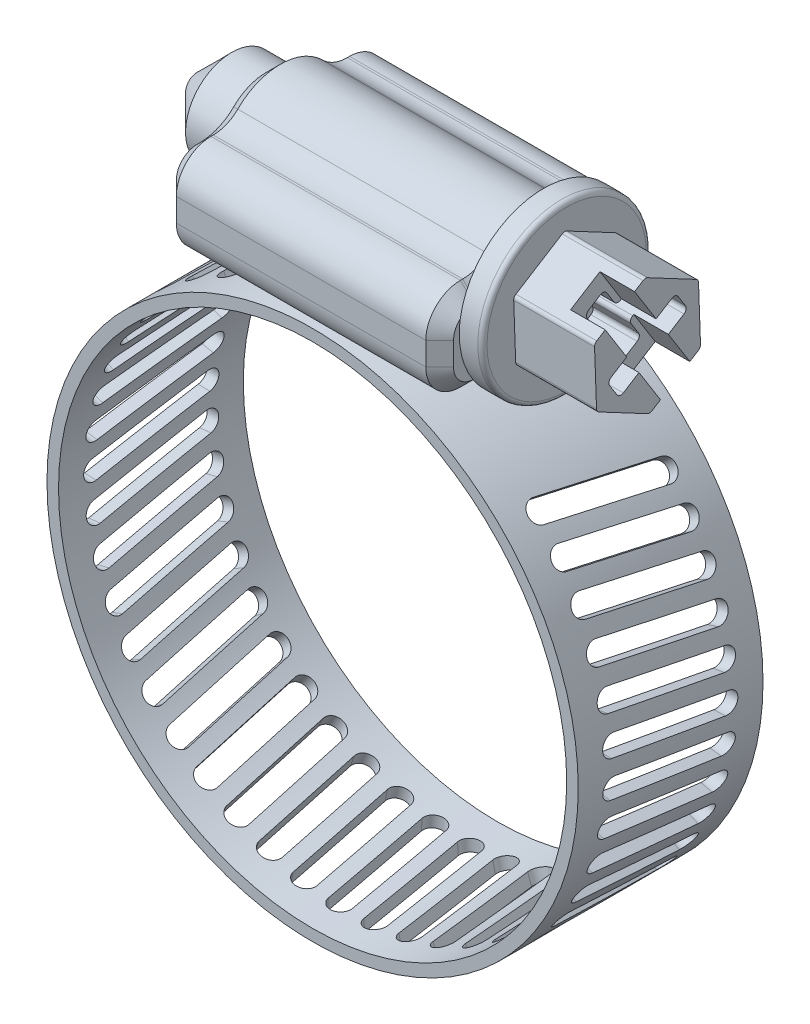
SolidWorks part; units mm, degrees
material "AISI 304"
ref_plane "Front Plane" through (0, 0, 0) normal (0, 0, 1) x (1, 0, 0)
ref_plane "Top Plane" through (0, 0, 0) normal (0, 1, 0) x (1, 0, 0)
ref_plane "Right Plane" through (0, 0, 0) normal (1, 0, 0) x (0, 0, -1)
sketch "Sketch1" plane through (0, 0, 0) normal (0, 0, 1) x (1, 0, 0)
  circle A0 centre (0, 0) radius 11
  dimension "D1" = 22
extrude "Extrude-Thin1" add sketch "Sketch1" along normal blind 8 thin
ref_plane "Plane1" through (0, 11.5, 0) normal (0, 1, 0) x (1, 0, 0)
ref_plane "Plane2" through (0, 0, 0) normal (1, 0, 0) x (0, 0, -1)
ref_plane "Plane3" through (6, 0, 0) normal (1, 0, 0) x (0, 0, -1)
sketch "Sketch2" plane through (6, 0, 0) normal (1, 0, 0) x (0, 0, -1)
  line L0 (-7, 11.5) -> (-1, 11.5)
  line L1 (6.765, 11.5) -> (-6.765, 11.5) construction
  line L2 (0.5, 13) -> (0.5, 14)
  line L3 (-1, 15.5) -> (-1.1, 15.5)
  line L4 (-8.5, 13) -> (-8.5, 14)
  line L5 (-7, 15.5) -> (-6.9, 15.5)
  line L6 (-8, 11.5) -> (-8, -11.5) construction
  line L7 (0, -11.5) -> (0, 11.5) construction
  arc A0 (-2.1608, 15.9395) -> (-5.8392, 15.9395) centre (-4, 14.1007) ccw
  arc A1 (0.5, 13) -> (-1, 11.5) centre (-1, 13) cw
  arc A2 (-8.5, 13) -> (-7, 11.5) centre (-7, 13) ccw
  arc A3 (-7, 15.5) -> (-8.5, 14) centre (-7, 14) ccw
  arc A4 (-1, 15.5) -> (0.5, 14) centre (-1, 14) cw
  arc A5 (-2.1608, 15.9395) -> (-1.1, 15.5) centre (-1.1, 17) ccw
  arc A6 (-5.8392, 15.9395) -> (-6.9, 15.5) centre (-6.9, 17) cw
  point P19 (0.5, 11.5)
  point P22 (-8.5, 11.5)
  dimension "D4" = 1.5
  dimension "D1" = 0.5
  dimension "D2" = 0.5
  dimension "D3" = 4
  dimension "D5" = 0.1
  dimension "D6" = 0.1
extrude "Boss-Extrude1" add sketch "Sketch2" against normal blind 12 separate body
sketch "Sketch3" plane through (6, 0, 0) normal (1, 0, 0) x (0, 0, -1)
  line L1 (-4.0935, 16.6997) -> (-6.2976, 15.3193)
  line L2 (-6.2976, 15.3193) -> (-6.2041, 12.7203)
  line L3 (-6.2041, 12.7203) -> (-3.9065, 11.5017)
  line L4 (-3.9065, 11.5017) -> (-1.7024, 12.8821)
  line L5 (-1.7024, 12.8821) -> (-1.7959, 15.4812)
  line L6 (-1.7959, 15.4812) -> (-4.0935, 16.6997)
  circle A1 centre (-4, 14.1007) radius 2.2523 construction
  arc A2 (-2.1608, 15.9395) -> (-5.8392, 15.9395) centre (-4, 14.1007) ccw construction
extrude "Boss-Extrude2" add sketch "Sketch3" along normal blind 4.5 separate body
chamfer "Chamfer1" distance 0.6 angle 45 24 edges at (6, 11.5, 4) (6, 11.9393, 8.0607) (6, 13.5, 8.5) (6, 15.0607, 8.0607) (6, 15.5, 6.95) (6, 15.6142, 6.3259) (6, 16.7014, 4) (6, 15.6142, 1.6741) (6, 15.5, 1.05) (6, 15.0607, -0.0607) (6, 13.5, -0.5) (6, 11.9393, -0.0607) (-6, 13.5, -0.5) (-6, 15.0607, -0.0607) (-6, 15.5, 1.05) (-6, 15.6142, 1.6741) (-6, 16.7014, 4) (-6, 15.6142, 6.3259) (-6, 15.5, 6.95) (-6, 15.0607, 8.0607) (-6, 13.5, 8.5) (-6, 11.9393, 8.0607) (-6, 11.5, 4) (-6, 11.9393, -0.0607)
fillet "Fillet1" radius 0.2 6 edges at (8.25, 11.5017, 3.9065) (8.25, 12.8821, 1.7024) (8.25, 15.4812, 1.7959) (8.25, 16.6997, 4.0935) (8.25, 12.7203, 6.2041) (8.25, 15.3193, 6.2976)
sketch "Sketch5" plane through (10.5, 0, 0) normal (1, 0, 0) x (0, 0, -1)
  line L0 (-5.8311, 15.6114) -> (-4.901, 14.1264)
  line L1 (-4.1913, 16.6385) -> (-6.1997, 15.3806) construction
  line L2 (-3.8087, 11.563) -> (-1.8003, 12.8209) construction
  line L3 (-3.4401, 11.7938) -> (-2.1689, 12.59)
  line L4 (-2.1689, 12.59) -> (-3.099, 14.0751)
  line L5 (-4.5599, 16.4076) -> (-5.8311, 15.6114)
  line L6 (-2.8045, 12.1919) -> (-5.1955, 16.0095) construction
  line L7 (-1.8221, 15.4648) -> (-6.1779, 12.7367) construction
  line L8 (-5.579, 13.7017) -> (-4.901, 14.1264)
  line L9 (-2.6761, 15.2839) -> (-2.3576, 14.7754)
  line L10 (-2.421, 14.4997) -> (-3.099, 14.0751)
  line L11 (-5.3239, 12.9176) -> (-5.6424, 13.4261)
  line L12 (-3.6298, 14.9226) -> (-2.9518, 15.3472)
  line L13 (-4.3702, 13.2789) -> (-3.4401, 11.7938)
  line L14 (-4.3702, 13.2789) -> (-5.0482, 12.8542)
  line L15 (-3.6298, 14.9226) -> (-4.5599, 16.4076)
  arc A0 (-1.7918, 15.3658) -> (-1.8979, 15.5353) centre (-1.9916, 15.3586) ccw construction
  arc A1 (-6.2082, 12.8356) -> (-6.1021, 12.6661) centre (-6.0084, 12.8428) ccw construction
  arc A2 (-5.579, 13.7017) -> (-5.6424, 13.4261) centre (-5.4729, 13.5322) ccw
  arc A3 (-5.3239, 12.9176) -> (-5.0482, 12.8542) centre (-5.1544, 13.0237) ccw
  arc A4 (-2.421, 14.4997) -> (-2.3576, 14.7754) centre (-2.5271, 14.6692) ccw
  arc A5 (-2.9518, 15.3472) -> (-2.6761, 15.2839) centre (-2.8456, 15.1777) cw
  point P25 (-5.7485, 13.5956)
  point P36 (-2.7823, 15.4534)
  dimension "D4" = 0.2
  dimension "D5" = 0.2
  dimension "D1" = 1.5
  dimension "D2" = 1
  dimension "D3" = 3.5
extrude "Cut-Extrude8" cut sketch "Sketch5" against normal blind 1.5
sketch "Sketch6" plane through (9, 0, 0) normal (1, 0, 0) x (0, 0, -1)
  line L0 (-4.901, 14.1264) -> (-5.579, 13.7017) construction
  line L1 (-2.9518, 15.3472) -> (-3.6722, 14.896)
  line L2 (-5.6424, 13.4261) -> (-5.3239, 12.9176) construction
  line L3 (-5.6424, 13.4261) -> (-5.3239, 12.9176)
  line L4 (-5.0482, 12.8542) -> (-4.3702, 13.2789) construction
  line L5 (-5.0482, 12.8542) -> (-4.3278, 13.3054)
  line L6 (-2.3576, 14.7754) -> (-2.6761, 15.2839) construction
  line L7 (-2.3576, 14.7754) -> (-2.6761, 15.2839)
  line L8 (-5.1138, 14.9371) -> (-4.7953, 14.4286)
  line L9 (-3.458, 12.6702) -> (-2.9495, 12.9887)
  line L10 (-2.8862, 13.2644) -> (-3.2047, 13.7729)
  line L11 (-4.542, 15.5312) -> (-5.0505, 15.2127)
  line L12 (-2.8045, 12.1919) -> (-8.6088, 21.4594) construction
  line L13 (-3.9478, 14.9594) -> (-4.2663, 15.4679)
  line L14 (-4.0522, 13.2421) -> (-3.7337, 12.7336)
  line L15 (-4.8586, 14.1529) -> (-5.579, 13.7017)
  line L16 (-3.1414, 14.0485) -> (-2.421, 14.4997)
  line L17 (-3.4401, 11.7938) -> (-2.1689, 12.59) construction
  arc A0 (-5.579, 13.7017) -> (-5.6424, 13.4261) centre (-5.4729, 13.5322) ccw construction
  arc A1 (-5.579, 13.7017) -> (-5.6424, 13.4261) centre (-5.4729, 13.5322) ccw
  arc A2 (-5.3239, 12.9176) -> (-5.0482, 12.8542) centre (-5.1544, 13.0237) ccw construction
  arc A3 (-5.3239, 12.9176) -> (-5.0482, 12.8542) centre (-5.1544, 13.0237) ccw
  arc A4 (-2.6761, 15.2839) -> (-2.9518, 15.3472) centre (-2.8456, 15.1777) ccw construction
  arc A5 (-2.6761, 15.2839) -> (-2.9518, 15.3472) centre (-2.8456, 15.1777) ccw
  arc A6 (-2.421, 14.4997) -> (-2.3576, 14.7754) centre (-2.5271, 14.6692) ccw construction
  arc A7 (-2.421, 14.4997) -> (-2.3576, 14.7754) centre (-2.5271, 14.6692) ccw
  arc A8 (-4.2663, 15.4679) -> (-4.542, 15.5312) centre (-4.4358, 15.3617) ccw
  arc A9 (-5.0505, 15.2127) -> (-5.1138, 14.9371) centre (-4.9443, 15.0432) ccw
  arc A10 (-2.8862, 13.2644) -> (-2.9495, 12.9887) centre (-3.0557, 13.1582) cw
  arc A11 (-3.7337, 12.7336) -> (-3.458, 12.6702) centre (-3.5642, 12.8397) ccw
  arc A12 (-3.1414, 14.0485) -> (-3.2047, 13.7729) centre (-3.0352, 13.879) ccw
  arc A13 (-4.3278, 13.3054) -> (-4.0522, 13.2421) centre (-4.2217, 13.1359) cw
  arc A14 (-3.9478, 14.9594) -> (-3.6722, 14.896) centre (-3.7783, 15.0655) ccw
  arc A15 (-4.7953, 14.4286) -> (-4.8586, 14.1529) centre (-4.9648, 14.3224) cw
  point P37 (-3.3109, 13.9424)
  point P44 (-4.6891, 14.2591)
  dimension "D1" = 0.2
  dimension "D2" = 0.2
  dimension "D5" = 0.2
  dimension "D3" = 1
  dimension "D4" = 3
extrude "Cut-Extrude9" cut sketch "Sketch6" against normal blind 2
sketch "Sketch7" plane through (-6, 0, 0) normal (-1, 0, 0) x (0, 0, 1)
  circle A0 centre (4, 14.1007) radius 2
  dimension "D1" = 4
extrude "Boss-Extrude3" add sketch "Sketch7" along normal blind 3
chamfer "Chamfer2" distance 1.5 angle 45 1 edges at (-9, 14.1007, 6)
sketch "Sketch8" plane through (6, 0, 0) normal (-1, 0, 0) x (0, 0, 1)
  circle A0 centre (4, 14.1007) radius 3.65
  dimension "D1" = 7.3
extrude "Boss-Extrude4" add sketch "Sketch8" against normal blind 1
fillet "Fillet3" radius 0.2 1 edges at (7, 14.1007, 7.65)
sketch "Sketch9" plane through (0, 11.5, 0) normal (0, -1, 0) x (1, 0, 0)
  line L0 (0.4341, 1.538) -> (-0.4341, 6.462) construction
  line L1 (-0.009, 1.4598) -> (-0.8773, 6.3839)
  line L2 (0.8773, 1.6161) -> (0.009, 6.5402)
  line L3 (-11, 0) -> (11, 0) construction
  line L4 (-11.5, 4) -> (21.4059, 4) construction
  line L5 (-11.5, 8) -> (-11.5, 0) construction
  line L6 (0, -0.5) -> (0, 14.6578) construction
  line L7 (-5.4, -0.5) -> (5.4, -0.5) construction
  arc A0 (-0.009, 1.4598) -> (0.8773, 1.6161) centre (0.4341, 1.538) ccw
  arc A1 (0.009, 6.5402) -> (-0.8773, 6.3839) centre (-0.4341, 6.462) ccw
  point P2 (0, 4)
  dimension "D1" = 100
  dimension "D2" = 0.9
  dimension "D3" = 5
extrude "Cut-Extrude10" cut sketch "Sketch9" along normal up to surface (0.535 mm away)
pattern_circular "CirPattern1" count 40 every 8 about axis through (0, 0, 0) along (0, 0, 1) of "Cut-Extrude10"
